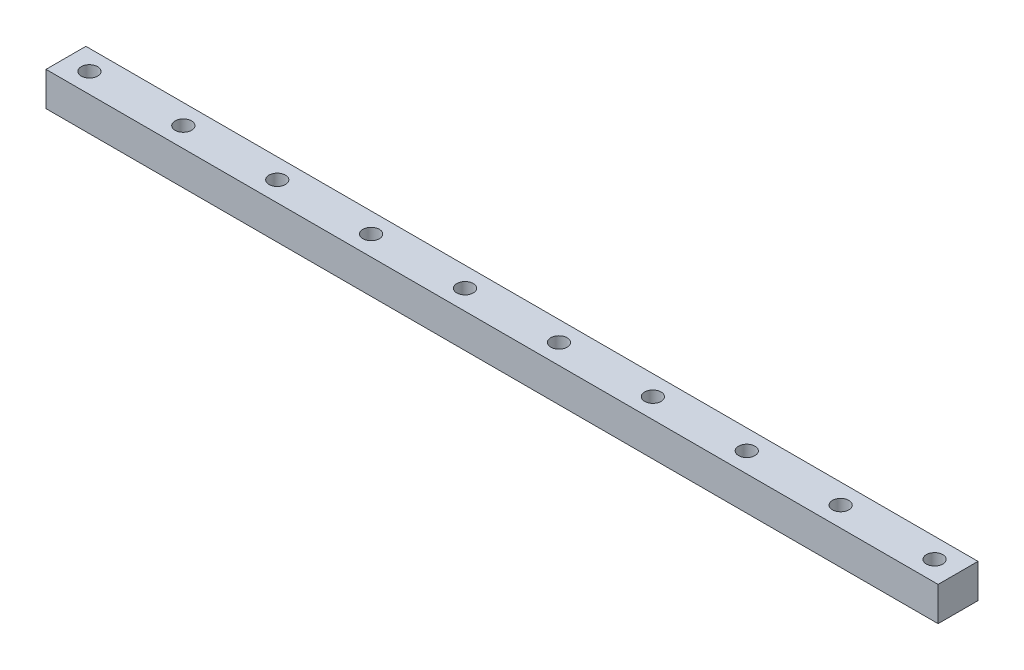
from build123d import *

# Parameters (mm, degrees)
SKETCH_1_W             = 760
SKETCH_1_H             = 34
EXTRUDE_1_DEPTH        = 29
SKETCH_2_R             = 7
CUT_EXTRUDE_1_DEPTH    = 12
SKETCH_3_R             = 4.5
CUT_EXTRUDE_2_DEPTH    = 761.950064065
PATTERN_LINEAR_1_COUNT = 10
PATTERN_LINEAR_1_PITCH = 80


with BuildPart() as part:
    # 草图1 → 拉伸1 (new body)
    with BuildSketch(Plane(origin=(0, 0, 0), x_dir=(1, 0, 0), z_dir=(0, 1, 0))):
        with Locations((380, 17)):
            Rectangle(SKETCH_1_W, SKETCH_1_H)
    extrude(amount=EXTRUDE_1_DEPTH)

    # 草图2 → 切除-拉伸1 (cut)
    with BuildSketch(Plane(origin=(0, 29, 0), x_dir=(-1, 0, 0), z_dir=(0, 1, 0))):
        with Locations(Location((-20, -17, 0), (0, 0, 90))):
            Circle(SKETCH_2_R)
    cut_extrude_1 = extrude(amount=-CUT_EXTRUDE_1_DEPTH, mode=Mode.SUBTRACT)

    # 草图3 → 切除-拉伸2 (cut, through all)
    with BuildSketch(Plane(origin=(0, 17, 0), x_dir=(-1, 0, 0), z_dir=(0, 1, 0))):
        with Locations(Location((-20, -17, 0), (0, 0, 90))):
            Circle(SKETCH_3_R)
    cut_extrude_2 = extrude(amount=-CUT_EXTRUDE_2_DEPTH, mode=Mode.SUBTRACT)

    # 阵列(线性)1: 切除-拉伸1, 切除-拉伸2 ×10
    with Locations(*[(i * PATTERN_LINEAR_1_PITCH, 0, 0) for i in range(1, PATTERN_LINEAR_1_COUNT)]):
        add(cut_extrude_1, mode=Mode.SUBTRACT)
        add(cut_extrude_2, mode=Mode.SUBTRACT)


solid = part.part
